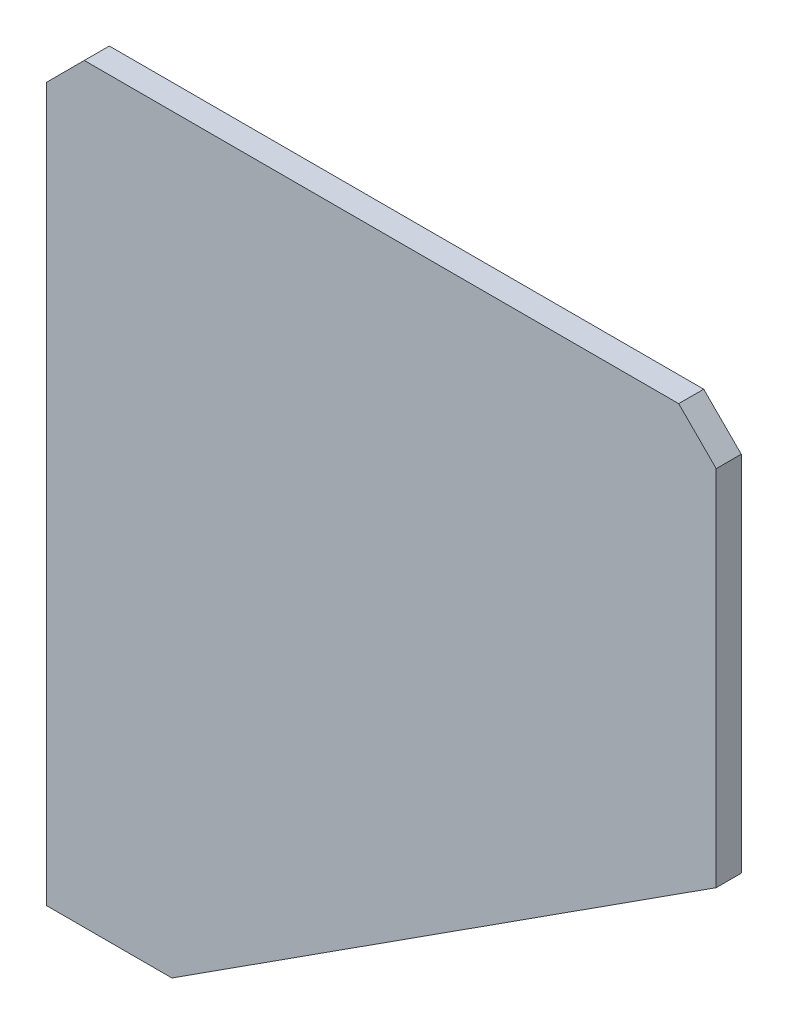
SolidWorks part; units mm, degrees
material "Q235-A"
ref_plane "前视基准面" through (0, 0, 0) normal (0, 0, 1) x (1, 0, 0)
ref_plane "上视基准面" through (0, 0, 0) normal (0, 1, 0) x (1, 0, 0)
ref_plane "右视基准面" through (0, 0, 0) normal (1, 0, 0) x (0, 0, -1)
sketch "草图1" plane through (0, 0, 0) normal (0, 0, 1) x (1, 0, 0)
  line L0 (0, 0) -> (53.5, 0)
  line L1 (53.5, 0) -> (53.5, -32)
  line L2 (53.5, -32) -> (10, -60)
  line L3 (10, -60) -> (0, -60)
  line L4 (0, -60) -> (0, 0)
  dimension "D1" = 53.5
  dimension "D2" = 60
  dimension "D3" = 32
  dimension "D4" = 10
extrude "凸台-拉伸1" add sketch "草图1" along normal blind 2
chamfer "倒角1" distance 3 angle 45 2 edges at (53.5, 0, 1) (0, 0, 1)
